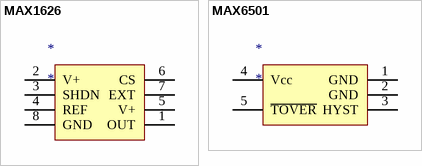
[diagram p0: symbols MAX1626 to MAX6501]
# Altium schematic symbol library MISC95141-2.SCHLIB: 2 symbols
Pins are listed as number, name and electrical type; pins without a type are passive.


## MAX1626
designator *
footprint DIP-4
pins: 1 OUT, 2 V+, 3 SHDN, 4 REF, 5 V+, 6 CS, 7 EXT, 8 GND

## MAX6501
designator *
footprint SO-G5/P.95
pins: 1 GND, 2 GND, 3 HYST, 4 Vcc, 5 ~{TOVER}